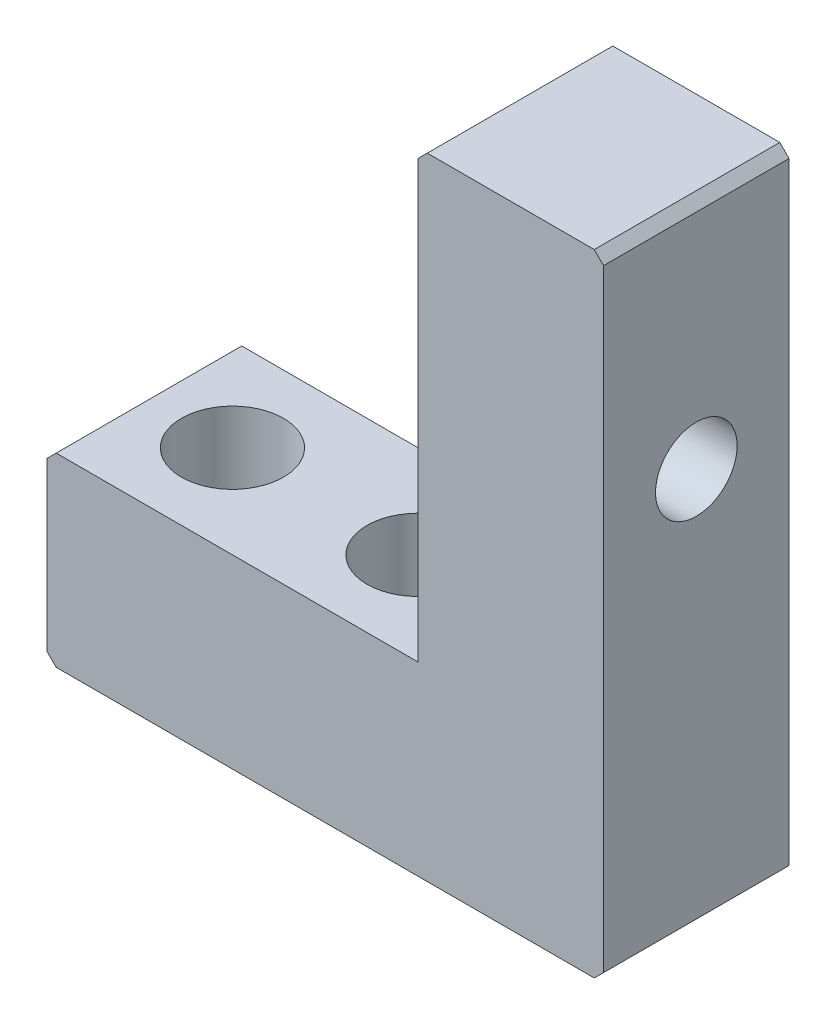
from build123d import *

# Parameters (mm, degrees)
BOSS_EXTRUDE1_DEPTH     = 20
M10X1_25_TAPPED_HOLE1_D = 8.8
HOLE1_D                 = 6.6
HOLE1_CBORE_D           = 11
HOLE1_CBORE_DEPTH       = 10
CHAMFER1_SIZE           = 1


with BuildPart() as part:
    # Sketch1 → Boss-Extrude1 (new body)
    with BuildSketch(Plane.XY):
        Polygon((6.43607117, 42.87394958), (6.43607117, -5.12605042), (-33.56392883, -5.12605042), (-33.56392883, -25.12605042), (26.43607117, -25.12605042), (26.43607117, 42.87394958), align=None)
    extrude(amount=BOSS_EXTRUDE1_DEPTH)

    # M10x1.25 Tapped Hole1 (through all)
    with Locations(Plane.ZY.offset(-6.43607117)):
        with Locations((10, 17.87394958)):
            Hole(M10X1_25_TAPPED_HOLE1_D / 2)

    # Hole1 (through all)
    with Locations(Plane(origin=(0, -5.12605042, 0), x_dir=(1, 0, 0), z_dir=(0, 1, 0))):
        with Locations((-3.56392883, -10), (-23.56392883, -10)):
            CounterBoreHole(HOLE1_D / 2, HOLE1_CBORE_D / 2, HOLE1_CBORE_DEPTH)

    # Chamfer1
    chamfer1_edges = [part.edges().sort_by_distance(p)[0] for p in [
        (26.43607117, 42.87394958, 10),
        (26.43607117, -25.12605042, 10),
        (-33.56392883, -25.12605042, 10),
        (-33.56392883, -5.12605042, 10),
        (6.43607117, 42.87394958, 10),
    ]]
    chamfer(chamfer1_edges, length=CHAMFER1_SIZE)


solid = part.part
